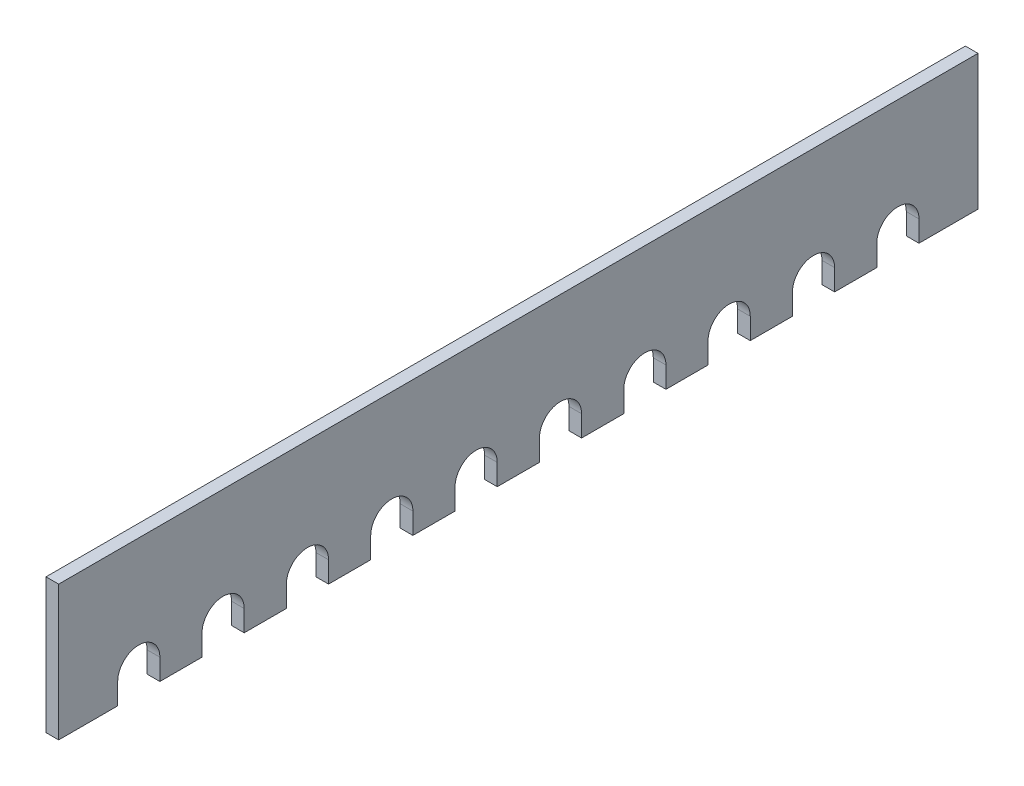
from build123d import *

# Parameters (mm, degrees)
SKETCH1_W           = 3
SKETCH1_H           = 32
EXTRUDE_THIN1_DEPTH = 218
CUT_EXTRUDE1_DEPTH  = 221.356529288
LPATTERN1_COUNT     = 10
LPATTERN1_PITCH     = 20


with BuildPart() as part:
    # Sketch1 → Extrude-Thin1 (new body)
    with BuildSketch(Plane.XY):
        with Locations((-1.5, -16)):
            Rectangle(SKETCH1_W, SKETCH1_H)
    extrude(amount=EXTRUDE_THIN1_DEPTH)

    # Sketch2 → Cut-Extrude1 (cut, through all)
    with BuildSketch(Plane(origin=(0, 0, 0), x_dir=(0, 0, -1), z_dir=(1, 0, 0))):
        with BuildLine():
            Line((-194, -27), (-194, -32))
            Line((-194, -32), (-204, -32))
            Line((-204, -32), (-204, -27))
            ThreePointArc((-204, -27), (-199, -22), (-194, -27))
        make_face()
    cut_extrude1 = extrude(amount=-CUT_EXTRUDE1_DEPTH, mode=Mode.SUBTRACT)

    # LPattern1: Cut-Extrude1 ×10
    with Locations(*[(0, 0, -i * LPATTERN1_PITCH) for i in range(1, LPATTERN1_COUNT)]):
        add(cut_extrude1, mode=Mode.SUBTRACT)


solid = part.part
